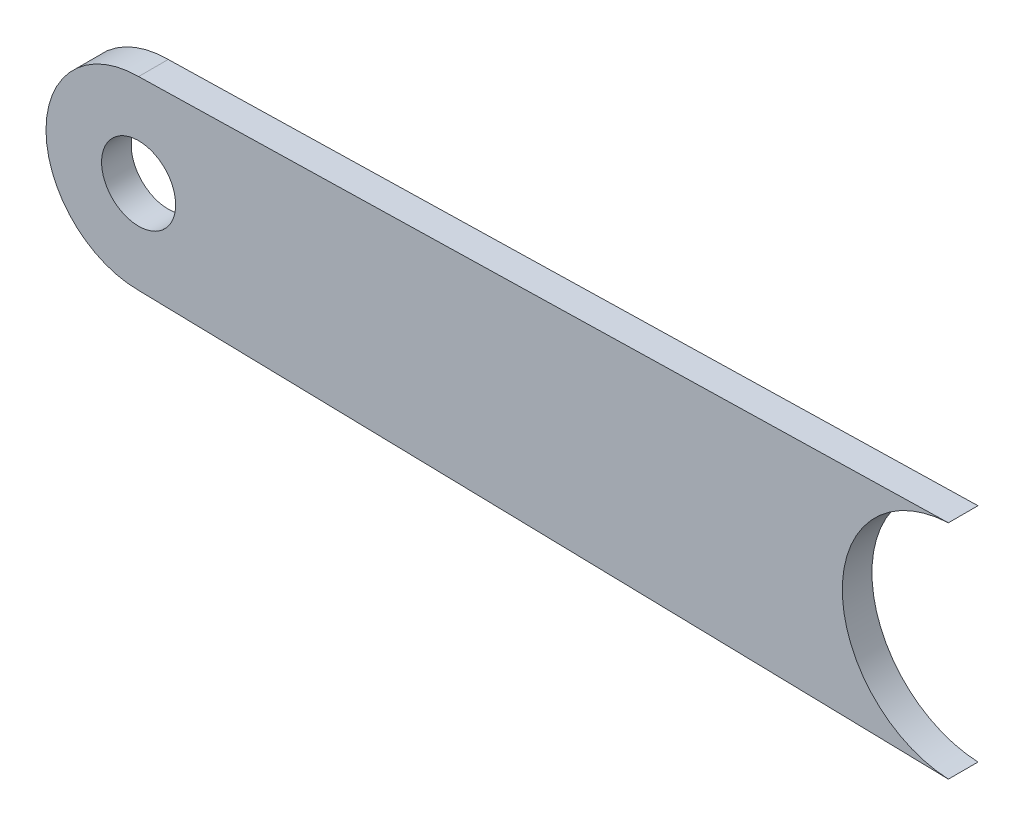
from build123d import *

# Parameters (mm, degrees)
EXTRUDE_1_DEPTH     = 8
SKETCH_2_R          = 10
CUT_EXTRUDE_1_DEPTH = 8


with BuildPart() as part:
    # 草图1 → 凸台-拉伸1 (new body)
    with BuildSketch(Plane.XY):
        with BuildLine():
            Line((218.63706763, 29.969024264), (0, 25))
            ThreePointArc((0, 25), (-25, 0), (0, -25))
            Line((0, -25), (218.63706763, -29.969024264))
            ThreePointArc((218.63706763, -29.969024264), (190, 0), (218.63706763, 29.969024264))
        make_face()
    extrude(amount=EXTRUDE_1_DEPTH)

    # 草图2 → 切除-拉伸1 (cut)
    with BuildSketch(Plane.XY.offset(8)):
        Circle(SKETCH_2_R)
    extrude(amount=-CUT_EXTRUDE_1_DEPTH, mode=Mode.SUBTRACT)


solid = part.part
